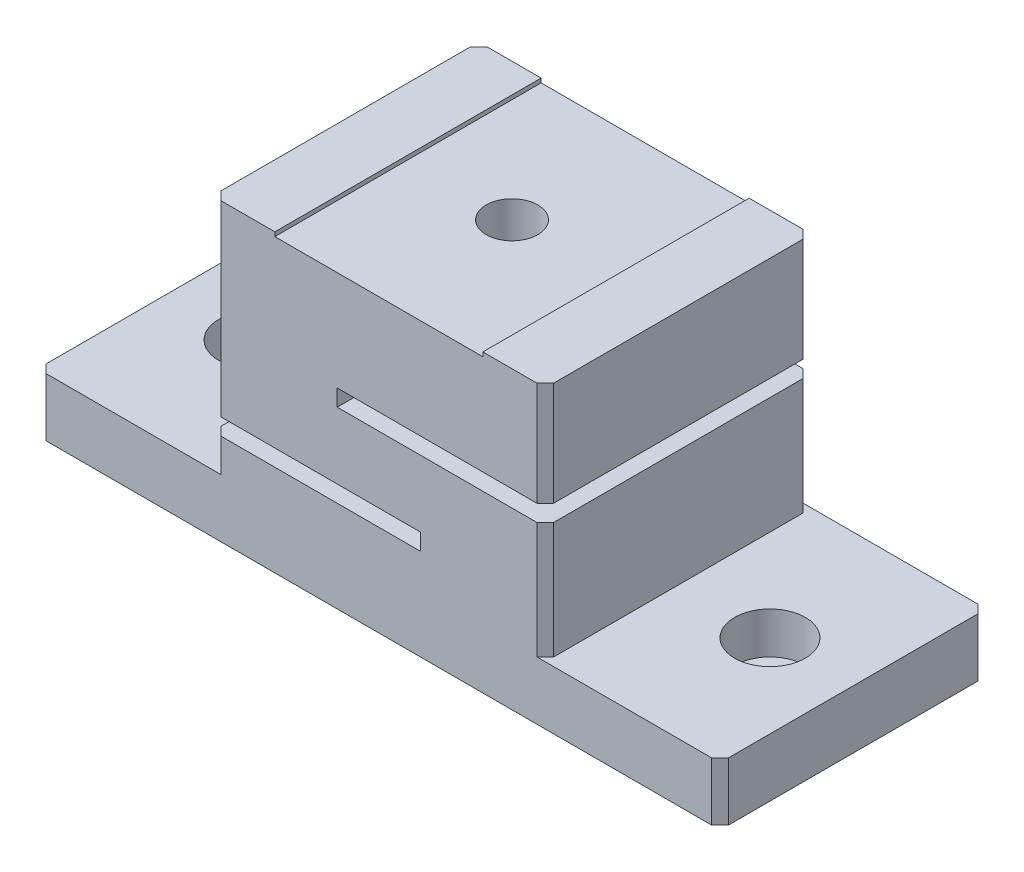
from build123d import *

# Parameters (mm, degrees)
SKETCH1_W           = 82
SKETCH1_H           = 32
BOSS_EXTRUDE1_DEPTH = 7
SKETCH2_W           = 40
SKETCH2_H           = 32
BOSS_EXTRUDE2_DEPTH = 28.5
SKETCH3_R           = 2.1
CUT_EXTRUDE1_DEPTH  = 28.5
SKETCH4_R           = 4.25
CUT_EXTRUDE2_DEPTH  = 5
SKETCH5_W           = 50
SKETCH5_H           = 2
SKETCH5_W_2         = 25
SKETCH5_H_2         = 1
CUT_EXTRUDE3_DEPTH  = 75
SKETCH6_R           = 6.5
CUT_EXTRUDE4_DEPTH  = 30
SKETCH7_R           = 3.1
CUT_EXTRUDE5_DEPTH  = 30
CHAMFER1_SIZE       = 1


with BuildPart() as part:
    # Sketch1 → Boss-Extrude1 (new body)
    with BuildSketch(Plane(origin=(0, 0, 0), x_dir=(1, 0, 0), z_dir=(0, 1, 0))):
        Rectangle(SKETCH1_W, SKETCH1_H)
    extrude(amount=BOSS_EXTRUDE1_DEPTH)

    # Sketch2 → Boss-Extrude2 (add)
    with BuildSketch(Plane(origin=(0, 7, 0), x_dir=(1, 0, 0), z_dir=(0, 1, 0))):
        Rectangle(SKETCH2_W, SKETCH2_H)
    extrude(amount=BOSS_EXTRUDE2_DEPTH)

    # Sketch3 → Cut-Extrude1 (cut)
    with BuildSketch(Plane(origin=(0, 7, 0), x_dir=(1, 0, 0), z_dir=(0, 1, 0))):
        with Locations(Location((31, 0, 0), (0, 0, 270))):
            Circle(SKETCH3_R)
        with Locations(Location((-31, 0, 0), (0, 0, 270))):
            Circle(SKETCH3_R)
    extrude(amount=-CUT_EXTRUDE1_DEPTH, mode=Mode.SUBTRACT)

    # Sketch4 → Cut-Extrude2 (cut)
    with BuildSketch(Plane(origin=(0, 7, 0), x_dir=(1, 0, 0), z_dir=(0, 1, 0))):
        with Locations(Location((-31, 0, 0), (0, 0, 270))):
            Circle(SKETCH4_R)
        with Locations(Location((31, 0, 0), (0, 0, 270))):
            Circle(SKETCH4_R)
    extrude(amount=-CUT_EXTRUDE2_DEPTH, mode=Mode.SUBTRACT)

    # Sketch5 → Cut-Extrude3 (cut)
    with BuildSketch(Plane(origin=(0, 0, -16), x_dir=(-1, 0, 0), z_dir=(0, 0, -1))):
        with Locations((20, 12)):
            Rectangle(SKETCH5_W, SKETCH5_H)
        with Locations((-20, 22)):
            Rectangle(SKETCH5_W, SKETCH5_H)
        with Locations((0, 35.5)):
            Rectangle(SKETCH5_W_2, SKETCH5_H_2)
    extrude(amount=-CUT_EXTRUDE3_DEPTH, mode=Mode.SUBTRACT)

    # Sketch6 → Cut-Extrude4 (cut)
    with BuildSketch(Plane.XZ):
        with Locations(Location((0, 0, 0), (0, 0, 270))):
            Circle(SKETCH6_R)
    extrude(amount=-CUT_EXTRUDE4_DEPTH, mode=Mode.SUBTRACT)

    # Sketch7 → Cut-Extrude5 (cut)
    with BuildSketch(Plane.XZ.offset(-30)):
        with Locations(Location((0, 0, 0), (0, 0, 270))):
            Circle(SKETCH7_R)
    extrude(amount=-CUT_EXTRUDE5_DEPTH, mode=Mode.SUBTRACT)

    # Chamfer1
    chamfer1_edges = [part.edges().sort_by_distance(p)[0] for p in [
        (20, 29.25, 16),
        (20, 29.25, -16),
        (-20, 24.25, -16),
        (-20, 24.25, 16),
        (-20, 9, 16),
        (-20, 9, -16),
        (20, 14, -16),
        (20, 14, 16),
        (41, 3.5, 16),
        (-41, 3.5, 16),
        (-41, 3.5, -16),
        (41, 3.5, -16),
    ]]
    chamfer(chamfer1_edges, length=CHAMFER1_SIZE)


solid = part.part
